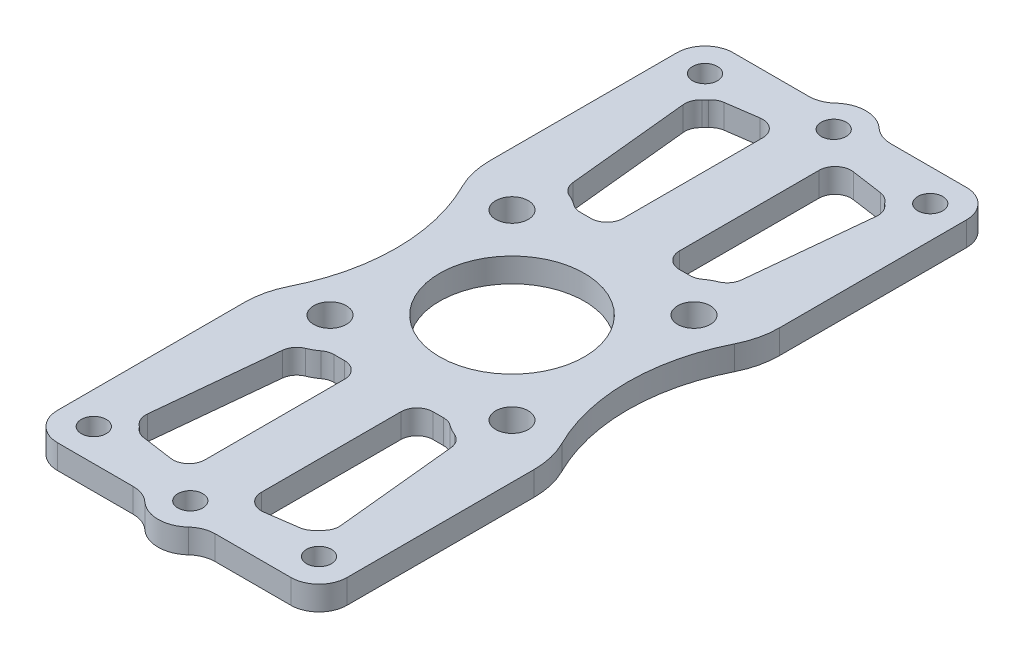
SolidWorks part; units mm, degrees
material "Thornel Mat VMA"
ref_plane "前视基准面" through (0, 0, 0) normal (0, 0, 1) x (1, 0, 0)
ref_plane "上视基准面" through (0, 0, 0) normal (0, 1, 0) x (1, 0, 0)
ref_plane "右视基准面" through (0, 0, 0) normal (1, 0, 0) x (0, 0, -1)
other "Configuration Table"
sketch "草图3" plane through (0, 0, 0) normal (0, 1, 0) x (1, 0, 0)
  line L0 (10, -34.1992) -> (10, 52.6309) construction
  line L1 (0, 0) -> (31.1432, 0) construction
  line L6 (-14, 38) -> (14, 38) construction
  line L7 (-14, 38) -> (-14, -38) construction
  line L8 (-14, -38) -> (14, -38) construction
  line L9 (14, 38) -> (14, -38) construction
  line L10 (-14, 38) -> (14, -38) construction
  line L11 (-14, -38) -> (14, 38) construction
  line L12 (-18, -42) -> (18, -42)
  line L13 (-18, -42) -> (-18, 42)
  line L14 (-18, 42) -> (18, 42)
  line L15 (18, -42) -> (18, 42)
  line L16 (-18, -42) -> (18, 42) construction
  line L17 (-18, 42) -> (18, -42) construction
  line L18 (0, 0) -> (11.3137, 11.3137) construction
  line L19 (0, 0) -> (0, -8.5999) construction
  circle A0 centre (0, 0) radius 16 construction
  circle A5 centre (0, 0) radius 9
  circle A6 centre (0, 0) radius 22 construction
  circle A7 centre (14, 38) radius 1.55
  circle A8 centre (-14, 38) radius 1.55
  circle A9 centre (-14, -38) radius 1.55
  circle A10 centre (14, -38) radius 1.55
  arc A11 (18, 12.6491) -> (18, -12.6491) centre (38.3961, 0) ccw
  arc A12 (-18, 12.6491) -> (-18, -12.6491) centre (-38.3961, 0) cw
  circle A15 centre (0, 40) radius 1.55
  circle A17 centre (0, 40) radius 4
  circle A19 centre (0, -40) radius 1.55
  circle A20 centre (0, -40) radius 4
  circle A21 centre (11.3137, 11.3137) radius 2.025
  circle A22 centre (11.3137, -11.3137) radius 2.025
  circle A23 centre (-11.3137, -11.3137) radius 2.025
  circle A24 centre (-11.3137, 11.3137) radius 2.025
  circle A25 centre (0, 0) radius 36 construction
  point P14 (0, 0)
  point P42 (0, 0)
  dimension "D1" = 32
  dimension "D2" = 45
  dimension "D4" = 18
  dimension "D5" = 44
  dimension "D9" = 3.1
  dimension "D12" = 4
  dimension "D13" = 8
  dimension "D14" = 2
  dimension "D15" = 4
  dimension "D3" = 4.05
  dimension "D16" = 24
  dimension "D17" = 72
  dimension "D6" = 10
  dimension "D7" = 4
  dimension "D8" = 76
  dimension "D10" = 28
  dimension "D11" = 4
extrude "凸台-拉伸1" add sketch "草图3" along normal blind 3
sketch "草图8" plane through (0, 3, 0) normal (0, 1, 0) x (1, 0, 0)
  line L0 (0, 0) -> (33.4914, 0) construction
  line L1 (-14, 38) -> (-11.3137, 11.3137)
  line L4 (-11.3137, 11.3137) -> (11.3137, 11.3137)
  line L7 (11.3137, 11.3137) -> (14, 38)
  line L10 (14, 38) -> (0, 40) construction
  line L13 (0, 40) -> (-14, 38) construction
  line L16 (0, 40) -> (0, 11.3137) construction
  line L19 (-3.5, 39.5) -> (-3.5, 15.3137)
  line L22 (3.5, 39.5) -> (3.5, 15.3137)
  line L25 (-11.3137, 11.3137) -> (11.3137, 11.3137) construction
  line L28 (-11.3137, 15.3137) -> (11.3137, 15.3137)
  line L31 (-11.3137, 7.3137) -> (11.3137, 7.3137)
  line L32 (-3.5, 39.5) -> (-3.5, 15.3137)
  line L33 (3.5, 39.5) -> (3.5, 15.3137)
  line L34 (0, 40) -> (14, 38) construction
  line L35 (-14, 38) -> (0, 40) construction
  line L36 (-11.3137, 11.3137) -> (-14, 38)
  line L37 (14, 38) -> (11.3137, 11.3137)
  line L38 (-14, 38) -> (-11.3137, 11.3137)
  line L39 (11.3137, 11.3137) -> (14, 38)
  line L40 (14, 38) -> (0, 40) construction
  line L41 (0, 40) -> (-14, 38) construction
  line L42 (-3.5, 39.5) -> (-3.5, 15.3137)
  line L43 (3.5, 39.5) -> (3.5, 15.3137)
  line L44 (-3.5, 39.5) -> (-3.5, 15.3137)
  line L45 (3.5, 39.5) -> (3.5, 15.3137)
  line L46 (0, 40) -> (14, 38)
  line L47 (-14, 38) -> (0, 40) construction
  line L48 (-11.3137, 11.3137) -> (-14, 38)
  line L49 (14, 38) -> (11.3137, 11.3137)
  line L50 (0, -40) -> (0, -11.3137) construction
  line L51 (14, -38) -> (11.3137, -11.3137)
  line L52 (-11.3137, -11.3137) -> (-14, -38)
  line L53 (0, -37.4746) -> (13.7494, -35.5104)
  line L54 (-13.7494, -35.5104) -> (0, -37.4746)
  line L55 (3.5, -39.5) -> (3.5, -15.3137)
  line L56 (-3.5, -39.5) -> (-3.5, -15.3137)
  line L57 (3.5, -39.5) -> (3.5, -15.3137)
  line L58 (-3.5, -39.5) -> (-3.5, -15.3137)
  line L59 (0, -40) -> (-14, -38) construction
  line L60 (14, -38) -> (0, -40) construction
  line L61 (11.3137, -11.3137) -> (14, -38)
  line L62 (-14, -38) -> (-11.3137, -11.3137)
  line L63 (14, -38) -> (11.3137, -11.3137)
  line L64 (-11.3137, -11.3137) -> (-14, -38)
  line L65 (-14, -38) -> (0, -40)
  line L66 (0, -40) -> (14, -38)
  line L67 (3.5, -39.5) -> (3.5, -15.3137)
  line L68 (-3.5, -39.5) -> (-3.5, -15.3137)
  line L69 (3.5, -39.5) -> (3.5, -15.3137)
  line L70 (-3.5, -39.5) -> (-3.5, -15.3137)
  line L71 (0, -40) -> (-14, -38)
  line L72 (14, -38) -> (0, -40)
  line L73 (11.3137, -11.3137) -> (14, -38)
  line L74 (-11.3137, -11.3137) -> (11.3137, -11.3137)
  line L75 (-14, -38) -> (-11.3137, -11.3137)
  line L76 (-11.3137, -11.3137) -> (11.3137, -11.3137) construction
  line L77 (-11.3137, -15.3137) -> (11.3137, -15.3137)
  line L78 (-11.3137, -7.3137) -> (11.3137, -7.3137)
  line L79 (-13.7494, 35.5104) -> (0, 37.4746)
  line L80 (0, 37.4746) -> (13.7494, 35.5104)
  line L81 (-12.1362, 34.4608) -> (-10.3512, 16.7288)
  line L82 (12.1362, 34.4608) -> (10.3512, 16.7288)
  line L83 (12.1362, -34.4608) -> (10.3512, -16.7288)
  line L84 (-12.1362, -34.4608) -> (-10.3512, -16.7288)
  circle A24 centre (-14, 38) radius 4
  circle A25 centre (14, 38) radius 4
  circle A26 centre (0, 0) radius 21 construction
  arc A27 (-11.3137, 15.3137) -> (-11.3137, 7.3137) centre (-11.3137, 11.3137) ccw
  arc A28 (11.3137, 7.3137) -> (11.3137, 15.3137) centre (11.3137, 11.3137) ccw
  circle A29 centre (-11.3137, 11.3137) radius 5.5
  circle A30 centre (11.3137, 11.3137) radius 5.5
  circle A31 centre (-11.3137, 11.3137) radius 5.5
  circle A32 centre (11.3137, 11.3137) radius 5.5
  circle A33 centre (-14, 38) radius 4
  circle A34 centre (14, 38) radius 4
  circle A35 centre (-14, 38) radius 4
  circle A36 centre (14, 38) radius 4
  circle A37 centre (-14, 38) radius 4
  circle A38 centre (14, 38) radius 4
  circle A39 centre (14, -38) radius 4
  circle A40 centre (-14, -38) radius 4
  circle A41 centre (14, -38) radius 4
  circle A42 centre (-14, -38) radius 4
  circle A43 centre (14, -38) radius 4
  circle A44 centre (-14, -38) radius 4
  circle A45 centre (11.3137, -11.3137) radius 5.5
  circle A46 centre (-11.3137, -11.3137) radius 5.5
  circle A47 centre (11.3137, -11.3137) radius 5.5
  circle A48 centre (-11.3137, -11.3137) radius 5.5
  circle A49 centre (14, -38) radius 4
  circle A50 centre (-14, -38) radius 4
  arc A51 (-11.3137, -15.3137) -> (-11.3137, -7.3137) centre (-11.3137, -11.3137) cw
  arc A52 (11.3137, -7.3137) -> (11.3137, -15.3137) centre (11.3137, -11.3137) cw
  point P18 (0, 11.3137)
  point P55 (0, -11.3137)
  dimension "D1" = 8
  dimension "D2" = 42
  dimension "D3" = 3.5
  dimension "D4" = 4
  dimension "D5" = 11
  dimension "D6" = 2.5
  dimension "D7" = 1.5
extrude "切除-拉伸2" cut sketch "草图8" against normal blind 3
fillet "圆角3" radius 2 24 edges at (7.5388, 1.5, -15.3137) (3.5, 1.5, -15.3137) (-3.5, 1.5, -15.3137) (-7.5388, 1.5, -15.3137) (3.5, 1.5, 15.3137) (7.5388, 1.5, 15.3137) (-7.5388, 1.5, 15.3137) (-3.5, 1.5, 15.3137) (10.5553, 1.5, -35.9667) (3.5, 1.5, -36.9746) (-3.5, 1.5, -36.9746) (-10.5553, 1.5, -35.9667) (10.5553, 1.5, 35.9667) (3.5, 1.5, 36.9746) (-3.5, 1.5, 36.9746) (-10.5553, 1.5, 35.9667) (12.1362, 1.5, 34.4608) (10.3512, 1.5, 16.7288) (12.1362, 1.5, -34.4608) (10.3512, 1.5, -16.7288) (-10.3512, 1.5, -16.7288) (-12.1362, 1.5, -34.4608) (-10.3512, 1.5, 16.7288) (-12.1362, 1.5, 34.4608)
fillet "圆角4" radius 3.5 8 edges at (18, 1.5, 42) (-18, 1.5, 42) (-18, 1.5, -42) (18, 1.5, -42) (3.4641, 1.5, 42) (-3.4641, 1.5, 42) (-3.4641, 1.5, -42) (3.4641, 1.5, -42)
fillet "圆角5" radius 10 4 edges at (18, 1.5, -12.6491) (18, 1.5, 12.6491) (-18, 1.5, 12.6491) (-18, 1.5, -12.6491)
